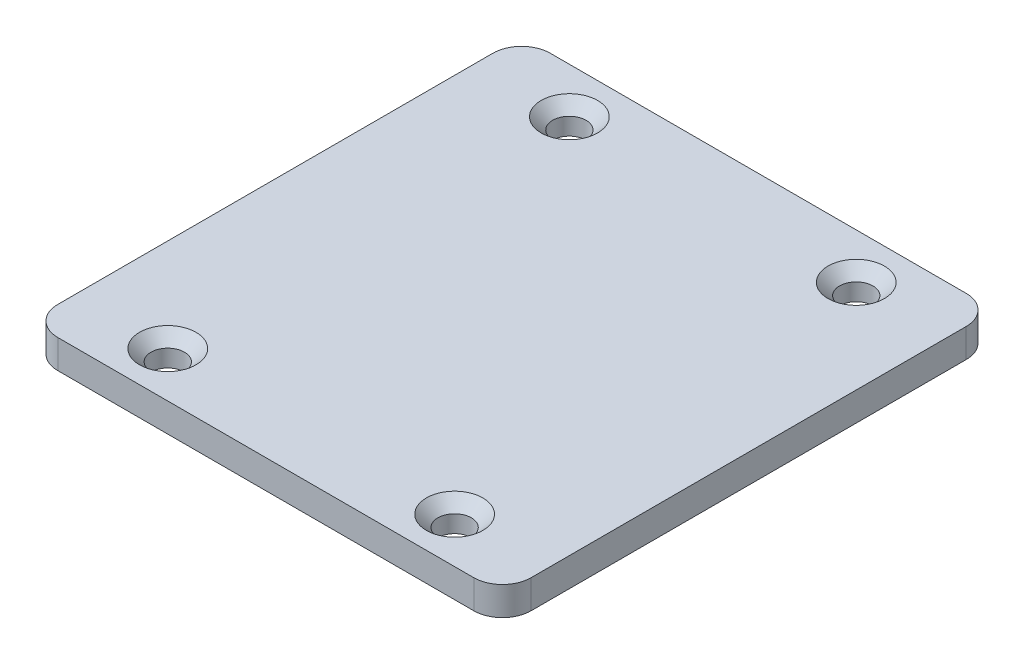
SolidWorks part; units mm, degrees
material "6061-T6 (SS)"
ref_plane "Front" through (0, 0, 0) normal (0, 0, 1) x (1, 0, 0)
ref_plane "Top" through (0, 0, 0) normal (0, 1, 0) x (1, 0, 0)
ref_plane "Right" through (0, 0, 0) normal (1, 0, 0) x (0, 0, -1)
sketch "Sketch1" plane through (0, 0, 0) normal (0, 1, 0) x (1, 0, 0)
  line L1 (-24.75, 25.75) -> (24.75, 25.75)
  line L2 (-24.75, 25.75) -> (-24.75, -25.75)
  line L3 (-24.75, -25.75) -> (24.75, -25.75)
  line L4 (24.75, 25.75) -> (24.75, -25.75)
  line L5 (-24.75, 25.75) -> (24.75, -25.75) construction
  line L6 (-24.75, -25.75) -> (24.75, 25.75) construction
  line L7 (-15, 21) -> (15, 21) construction
  line L8 (-15, 21) -> (-15, -21) construction
  line L9 (-15, -21) -> (15, -21) construction
  line L10 (15, 21) -> (15, -21) construction
  line L11 (-15, 21) -> (15, -21) construction
  line L12 (-15, -21) -> (15, 21) construction
  circle A0 centre (-15, 21) radius 1.75
  circle A1 centre (15, 21) radius 1.75
  circle A2 centre (-15, -21) radius 1.75
  circle A3 centre (15, -21) radius 1.75
  point P0 (0, 0)
  point P6 (0, 0)
  dimension "D5" = 3.5
  dimension "D1" = 49.5
  dimension "D2" = 51.5
  dimension "D3" = 30
  dimension "D4" = 42
extrude "Boss-Extrude1" add sketch "Sketch1" along normal blind 3
chamfer "Chamfer1" distance 1.2 angle 45 4 edges at (-15, 3, 22.75) (15, 3, 22.75) (15, 3, -19.25) (-15, 3, -19.25)
fillet "Fillet1" radius 3 4 edges at (-24.75, 1.5, 25.75) (-24.75, 1.5, -25.75) (24.75, 1.5, -25.75) (24.75, 1.5, 25.75)
